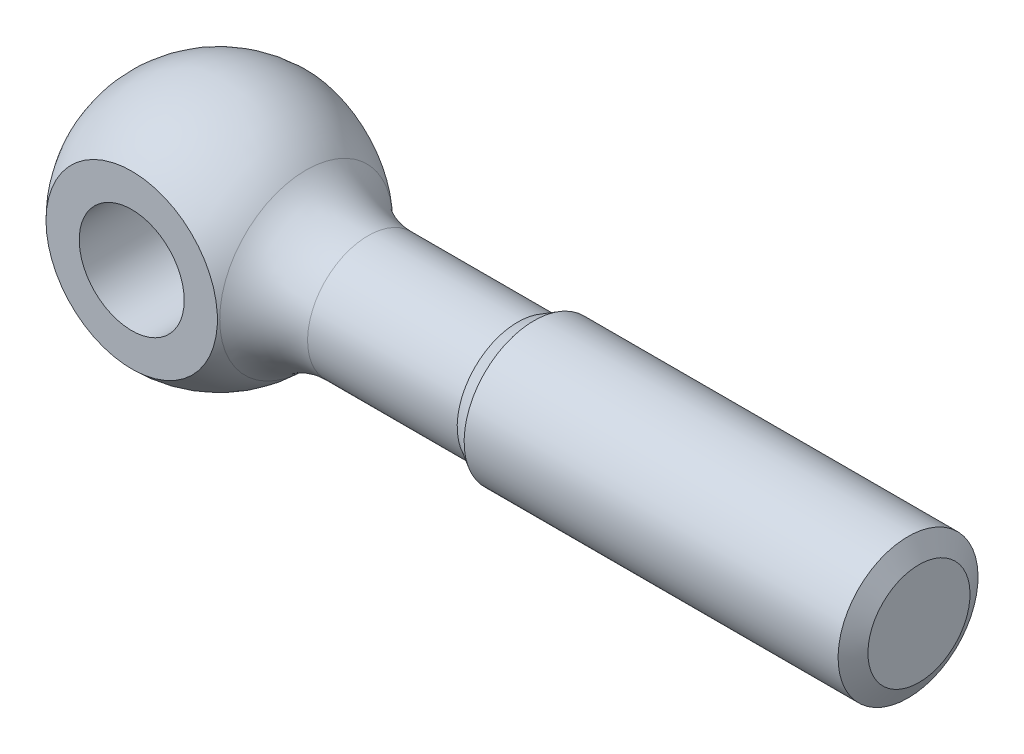
from build123d import *
from build123d.topology import SkipClean

# Parameters (mm, degrees)
CUT_EXTRUDE1_DEPTH      = 13.124356
CUT_EXTRUDE1_DEPTH_BACK = 13.124356
SKETCH4_R               = 3
CUT_EXTRUDE2_DEPTH      = 16.556349
CHAMFER1_SIZE           = 0.4
FILLET1_R               = 5


with BuildPart() as part:
    # Sketch1 → Boss-Revolve (revolve)
    with BuildSketch(Plane.XY):
        with BuildLine():
            Line((-7, 0), (7, 0))
            ThreePointArc((7, 0), (0, 7), (-7, 0))
        make_face()
    revolve(axis=Axis((-13.286843, 0, 0), (1, 0, 0)))

    # Sketch2 → Cut-Extrude1 (cut, two sides: drawn at the far end of the back side and taken through both)
    with SkipClean():  # the faces are left unmerged after this step: merging them gives an invalid solid
        with BuildSketch(Plane(origin=(0, 0, 0), x_dir=(0, 0, -1), z_dir=(1, 0, 0)).offset(-CUT_EXTRUDE1_DEPTH_BACK)):
            with BuildLine():
                Line((-5, 4.898979), (-5, -4.898979))
                ThreePointArc((-5, -4.898979), (-7, 0), (-5, 4.898979))
            make_face()
            with BuildLine():
                Line((5, 4.898979), (5, -4.898979))
                ThreePointArc((5, -4.898979), (7, 0), (5, 4.898979))
            make_face()
        extrude(amount=CUT_EXTRUDE1_DEPTH + CUT_EXTRUDE1_DEPTH_BACK, mode=Mode.SUBTRACT)

    # Sketch4 → Cut-Extrude2 (cut, through all)
    with SkipClean():  # the faces are left unmerged after this step: merging them gives an invalid solid
        with BuildSketch(Plane.XY.offset(5)):
            Circle(SKETCH4_R)
        extrude(amount=-CUT_EXTRUDE2_DEPTH, mode=Mode.SUBTRACT)

    # Sketch5 → Boss-Revolve1 (revolve)
    with SkipClean():  # the faces are left unmerged after this step: merging them gives an invalid solid
        with BuildSketch(Plane.XY, mode=Mode.PRIVATE) as boss_revolve1_sk:
            Polygon((3.469445, 3.45875), (3.469445, 0), (40, 0), (40, 4), (18, 4), (17.062528, 3.45875), align=None)
        revolve(boss_revolve1_sk.sketch.rotate(Axis((0, 0, 0), (1, 0, 0)), 180), axis=Axis((0, 0, 0), (1, 0, 0)))

    # Chamfer1
    chamfer1_edges = [part.edges().sort_by_distance(p)[0] for p in [
        (40, 4, 0),
    ]]
    chamfer(chamfer1_edges, length=CHAMFER1_SIZE)

    # Sketch6 → Cut-Revolve1 (revolve, cut)
    with SkipClean():  # the faces are left unmerged after this step: merging them gives an invalid solid
        with BuildSketch(Plane.XY, mode=Mode.PRIVATE) as cut_revolve1_sk:
            Polygon((39.375018, 4), (40.624982, 4), (40, 2.9175), align=None)
        revolve(cut_revolve1_sk.sketch.rotate(Axis((0, 0, 0), (1, 0, 0)), 180), axis=Axis((0, 0, 0), (1, 0, 0)), mode=Mode.SUBTRACT)

    # Fillet1
    fillet1_edges = [part.edges().sort_by_distance(p)[0] for p in [
        (6.085807, 0, -3.45875),
    ]]
    fillet(fillet1_edges, radius=FILLET1_R)


solid = part.part
